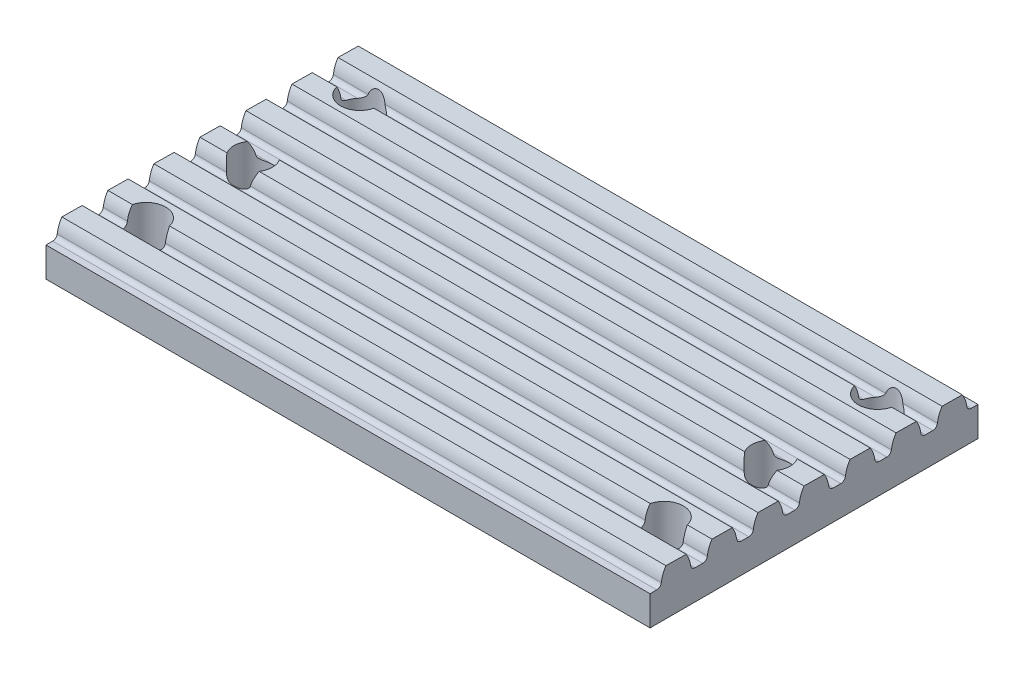
SolidWorks part; units mm, degrees
material "A6061"
ref_plane "前基準面" through (0, 0, 0) normal (0, 0, 1) x (1, 0, 0)
ref_plane "上基準面" through (0, 0, 0) normal (0, 1, 0) x (1, 0, 0)
ref_plane "右基準面" through (0, 0, 0) normal (1, 0, 0) x (0, 0, -1)
sketch "草图1" plane through (0, 0, 0) normal (0, 0, 1) x (1, 0, 0)
  line L0 (0, 0) -> (105, 0)
  dimension "D1" = 105
other "其他 S8M压板(1)"
ref_plane "基准面1" through (0, 0, -28.5) normal (1, 0, 0) x (0, 0, -1)
sketch "草图12" plane through (0, 0, -28.5) normal (1, 0, 0) x (0, 0, -1)
  line L0 (0, 0) -> (0, 18.485) construction
  line L1 (0, 0) -> (34.5949, 0) construction
  line L36 (-27.3463, 5.15) -> (-28.5, 5.15)
  line L37 (-28.5, 5.15) -> (-28.5, 0)
  line L38 (-28.5, 0) -> (28.5, 0)
  line L39 (28.5, 0) -> (28.5, 5.15)
  line L40 (28.5, 5.15) -> (27.3458, 5.15)
  line L41 (25.779, 7.954) -> (22.2507, 7.9998)
  line L42 (20.6537, 5.15) -> (19.3458, 5.15)
  line L43 (17.779, 7.954) -> (14.2507, 7.9998)
  line L44 (12.6537, 5.15) -> (11.3458, 5.15)
  line L45 (9.779, 7.954) -> (6.2507, 7.9998)
  line L46 (4.6537, 5.15) -> (3.3458, 5.15)
  line L47 (1.779, 7.954) -> (-1.7493, 7.9998)
  line L48 (-3.3463, 5.15) -> (-4.6542, 5.15)
  line L49 (-6.221, 7.954) -> (-9.7493, 7.9998)
  line L50 (-11.3463, 5.15) -> (-12.6542, 5.15)
  line L51 (-14.221, 7.954) -> (-17.7493, 7.9998)
  line L52 (-19.3463, 5.15) -> (-20.6542, 5.15)
  line L53 (-22.221, 7.954) -> (-25.7493, 7.9998)
  arc A56 (-25.7493, 7.9998) -> (-26.5535, 5.8433) centre (-21.3999, 5.1498) ccw
  arc A57 (-27.3463, 5.15) -> (-26.5535, 5.8433) centre (-27.3463, 5.95) ccw
  arc A58 (26.5529, 5.8434) -> (27.3458, 5.15) centre (27.3458, 5.95) ccw
  arc A59 (26.5529, 5.8434) -> (25.779, 7.954) centre (21.3993, 5.1508) ccw
  arc A60 (22.2507, 7.9998) -> (21.4465, 5.8433) centre (26.6001, 5.1498) ccw
  arc A61 (20.6537, 5.15) -> (21.4465, 5.8433) centre (20.6537, 5.95) ccw
  arc A62 (18.5529, 5.8434) -> (19.3458, 5.15) centre (19.3458, 5.95) ccw
  arc A63 (18.5529, 5.8434) -> (17.779, 7.954) centre (13.3993, 5.1508) ccw
  arc A64 (14.2507, 7.9998) -> (13.4465, 5.8433) centre (18.6001, 5.1498) ccw
  arc A65 (12.6537, 5.15) -> (13.4465, 5.8433) centre (12.6537, 5.95) ccw
  arc A66 (10.5529, 5.8434) -> (11.3458, 5.15) centre (11.3458, 5.95) ccw
  arc A67 (10.5529, 5.8434) -> (9.779, 7.954) centre (5.3993, 5.1508) ccw
  arc A68 (6.2507, 7.9998) -> (5.4465, 5.8433) centre (10.6001, 5.1498) ccw
  arc A69 (4.6537, 5.15) -> (5.4465, 5.8433) centre (4.6537, 5.95) ccw
  arc A70 (2.5529, 5.8434) -> (3.3458, 5.15) centre (3.3458, 5.95) ccw
  arc A71 (2.5529, 5.8434) -> (1.779, 7.954) centre (-2.6007, 5.1508) ccw
  arc A72 (-1.7493, 7.9998) -> (-2.5535, 5.8433) centre (2.6001, 5.1498) ccw
  arc A73 (-3.3463, 5.15) -> (-2.5535, 5.8433) centre (-3.3463, 5.95) ccw
  arc A74 (-5.4471, 5.8434) -> (-4.6542, 5.15) centre (-4.6542, 5.95) ccw
  arc A75 (-5.4471, 5.8434) -> (-6.221, 7.954) centre (-10.6007, 5.1508) ccw
  arc A76 (-9.7493, 7.9998) -> (-10.5535, 5.8433) centre (-5.3999, 5.1498) ccw
  arc A77 (-11.3463, 5.15) -> (-10.5535, 5.8433) centre (-11.3463, 5.95) ccw
  arc A78 (-13.4471, 5.8434) -> (-12.6542, 5.15) centre (-12.6542, 5.95) ccw
  arc A79 (-13.4471, 5.8434) -> (-14.221, 7.954) centre (-18.6007, 5.1508) ccw
  arc A80 (-17.7493, 7.9998) -> (-18.5535, 5.8433) centre (-13.3999, 5.1498) ccw
  arc A81 (-19.3463, 5.15) -> (-18.5535, 5.8433) centre (-19.3463, 5.95) ccw
  arc A82 (-21.4471, 5.8434) -> (-20.6542, 5.15) centre (-20.6542, 5.95) ccw
  arc A83 (-21.4471, 5.8434) -> (-22.221, 7.954) centre (-26.6007, 5.1508) ccw
  point P19 (0, 0)
hole_wizard "M6 间隙孔1" positions "草图13" profile "草图14" hole size "M6" standard "GB" end condition through all
sketch "草图13" plane through (0, 0, 0) normal (0, -1, 0) x (-1, 0, 0)
  line L0 (-52.5, 0) -> (-52.5, 61.4623) construction
  line L1 (-105, 0) -> (0, 0) construction
  line L3 (0, 28.5) -> (-115.0618, 28.5) construction
  line L5 (-105, 57) -> (0, 57) construction
  line L6 (0, 0) -> (0, 57) construction
  point P0 (-7.5, 10)
  point P2 (-7.5, 47)
  point P16 (-97.5, 47)
  point P17 (-97.5, 10)
  point P27 (-97.5, 28.5)
  point P29 (-7.5, 28.5)
  dimension "D1" = 10
  dimension "D2" = 7.5
  dimension "D3" = 10
  dimension "D4" = 90
  dimension "D5" = 37
sketch "草图14" plane through (7.5, 0, -10) normal (1, 0, 0) x (0, 0, -1)
  line L0 (0, 0) -> (0, 7.9998)
  line L1 (0, 7.9998) -> (3.3, 7.9998)
  line L2 (3.3, 7.9998) -> (3.3, 0)
  line L5 (3.3, 0) -> (0, 0)
  line L11 (0, -6.35) -> (0, 107.95) construction
  dimension "通孔孔直径" = 6.6
  dimension "通孔孔深度" = 7.9998
